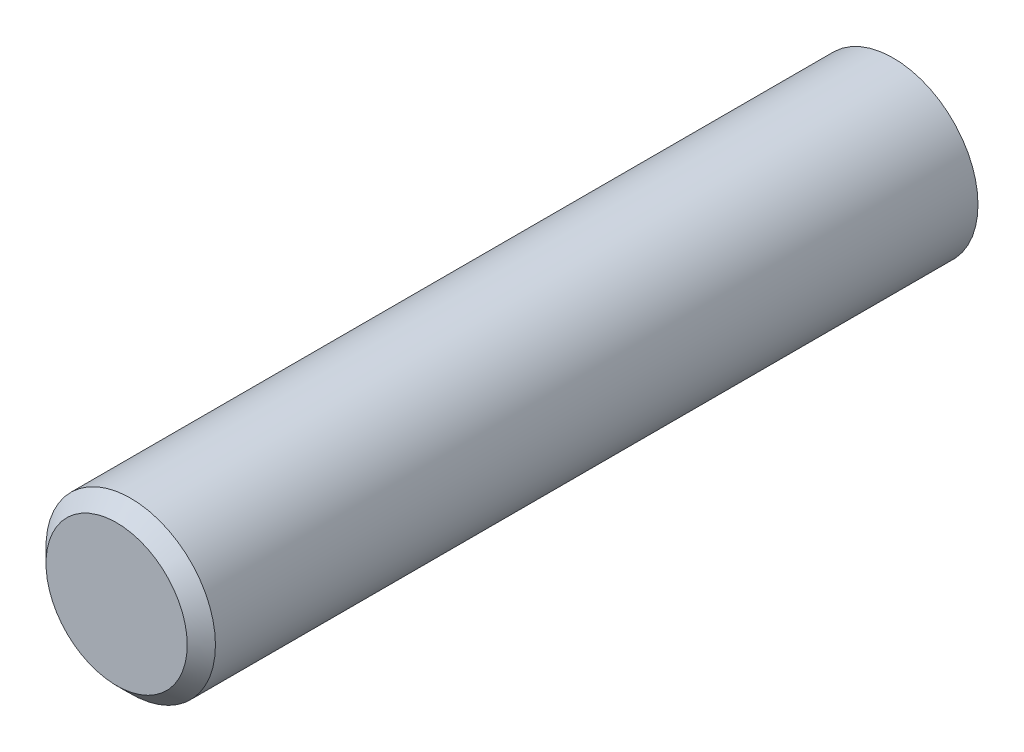
from build123d import *

# Parameters (mm, degrees)
SKETCH1_R           = 6
BOSS_EXTRUDE1_DEPTH = 55
CHAMFER1_SIZE       = 1


with BuildPart() as part:
    # Sketch1 → Boss-Extrude1 (new body)
    with BuildSketch(Plane.XY):
        Circle(SKETCH1_R)
    extrude(amount=BOSS_EXTRUDE1_DEPTH)

    # Chamfer1
    chamfer1_edges = [part.edges().sort_by_distance(p)[0] for p in [
        (-6, 0, 55),
    ]]
    chamfer(chamfer1_edges, length=CHAMFER1_SIZE)


solid = part.part
